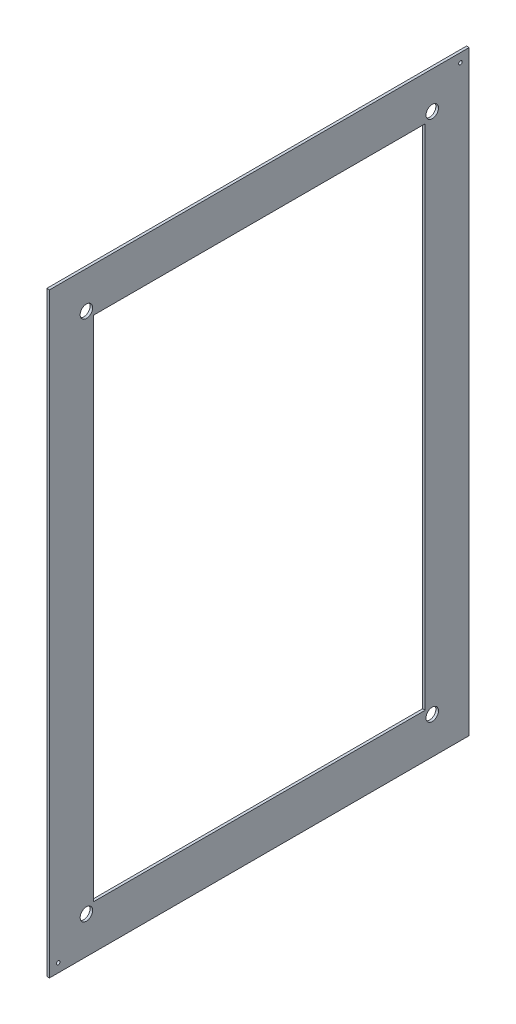
SolidWorks part; units mm, degrees
ref_plane "前视基准面" through (0, 0, 0) normal (0, 0, 1) x (1, 0, 0)
ref_plane "上视基准面" through (0, 0, 0) normal (0, 1, 0) x (1, 0, 0)
ref_plane "右视基准面" through (0, 0, 0) normal (1, 0, 0) x (0, 0, -1)
ref_plane "基准面4" through (2615.9295, 0, 0) normal (1, 0, 0) x (0, 0, -1)
sketch "草图1" plane through (2615.9295, 0, 0) normal (1, 0, 0) x (0, 0, -1)
  line L0 (-285.1446, 1066.7) -> (-285.1446, 1355.3)
  line L1 (-285.1446, 1355.3) -> (-96.6446, 1355.3)
  line L2 (-96.6446, 1355.3) -> (-96.6446, 1066.7)
  line L3 (-96.6446, 1066.7) -> (-285.1446, 1066.7)
  line L4 (-310.1446, 1041.7) -> (-71.6446, 1041.7)
  line L5 (-71.6446, 1041.7) -> (-71.6446, 1380.3)
  line L6 (-71.6446, 1380.3) -> (-310.1446, 1380.3)
  line L7 (-310.1446, 1380.3) -> (-310.1446, 1041.7)
  circle A0 centre (-305.1446, 1046.7) radius 1
  circle A1 centre (-76.6446, 1375.3) radius 1
  circle A2 centre (-289.1446, 1062.7) radius 3.55
  circle A3 centre (-92.6446, 1359.3) radius 3.55
  circle A4 centre (-92.6446, 1062.7) radius 3.55
  circle A5 centre (-289.1446, 1359.3) radius 3.55
extrude "凸台-拉伸1" add sketch "草图1" against normal blind 1.5
